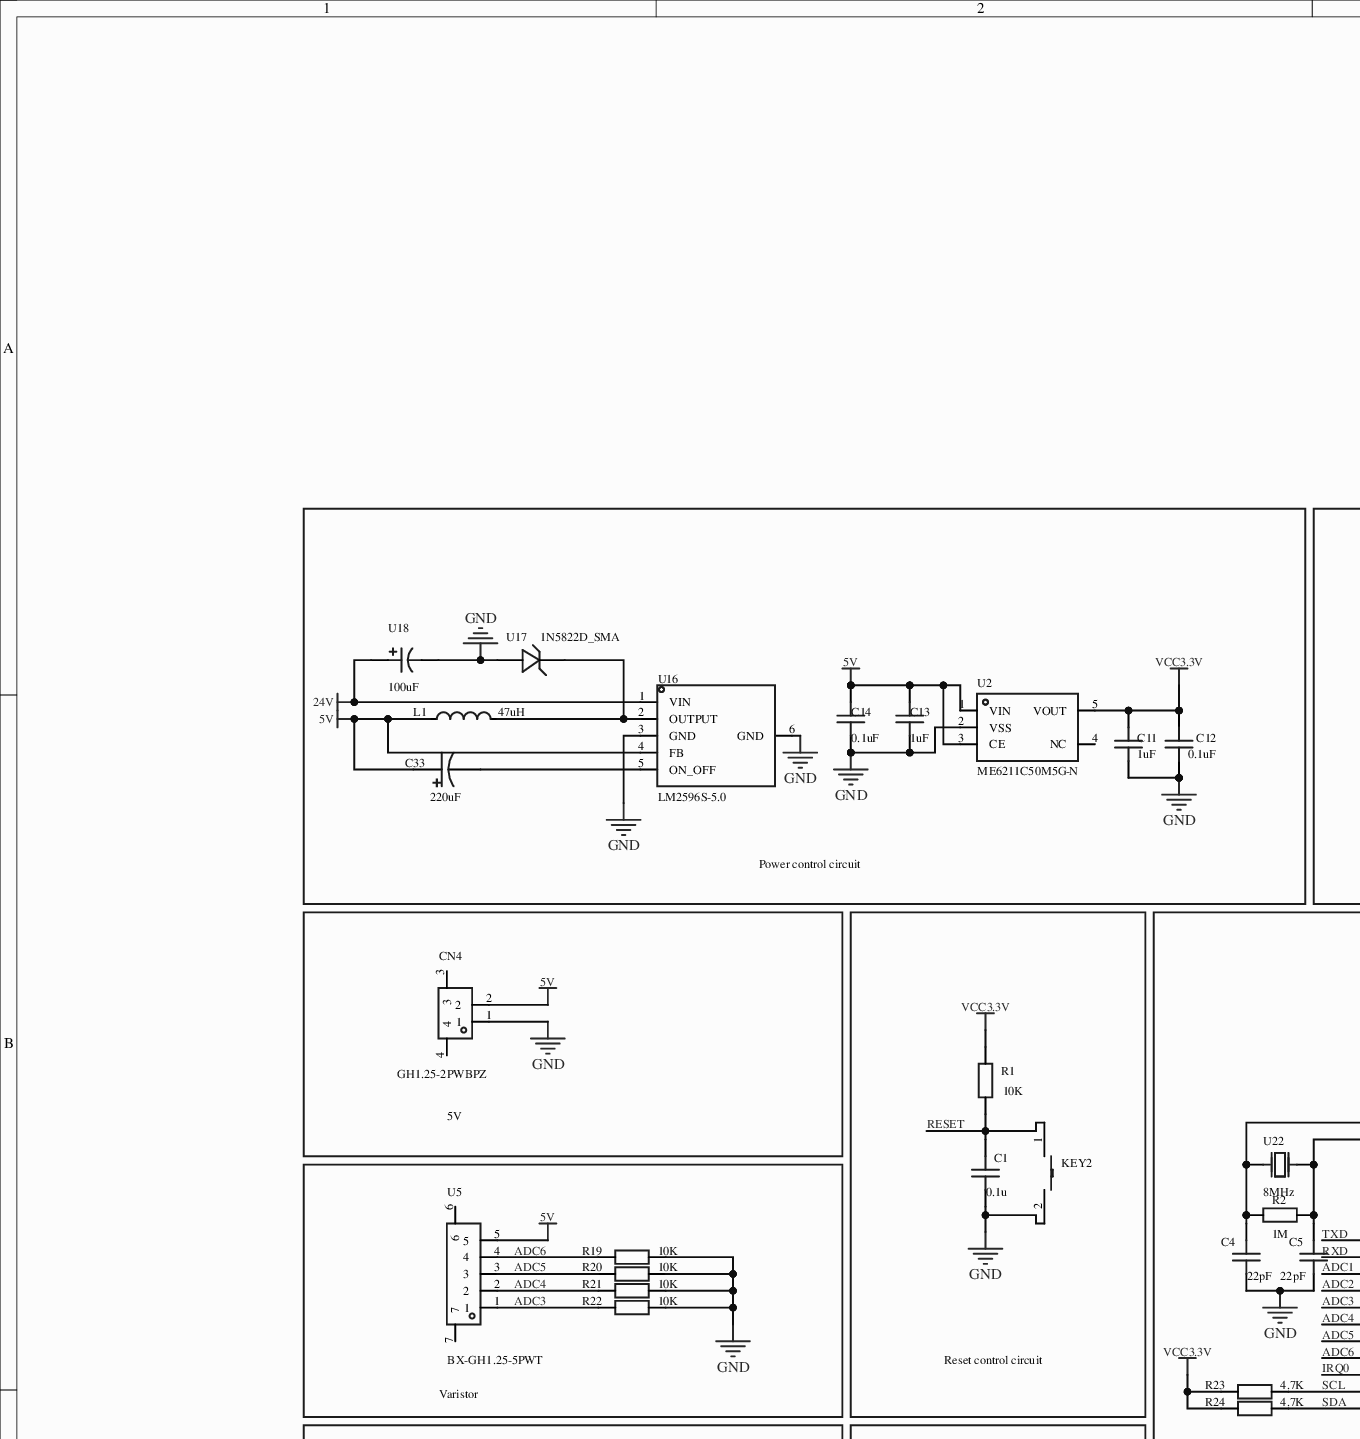
[diagram p0: MISC61403-3.schdoc, top left]
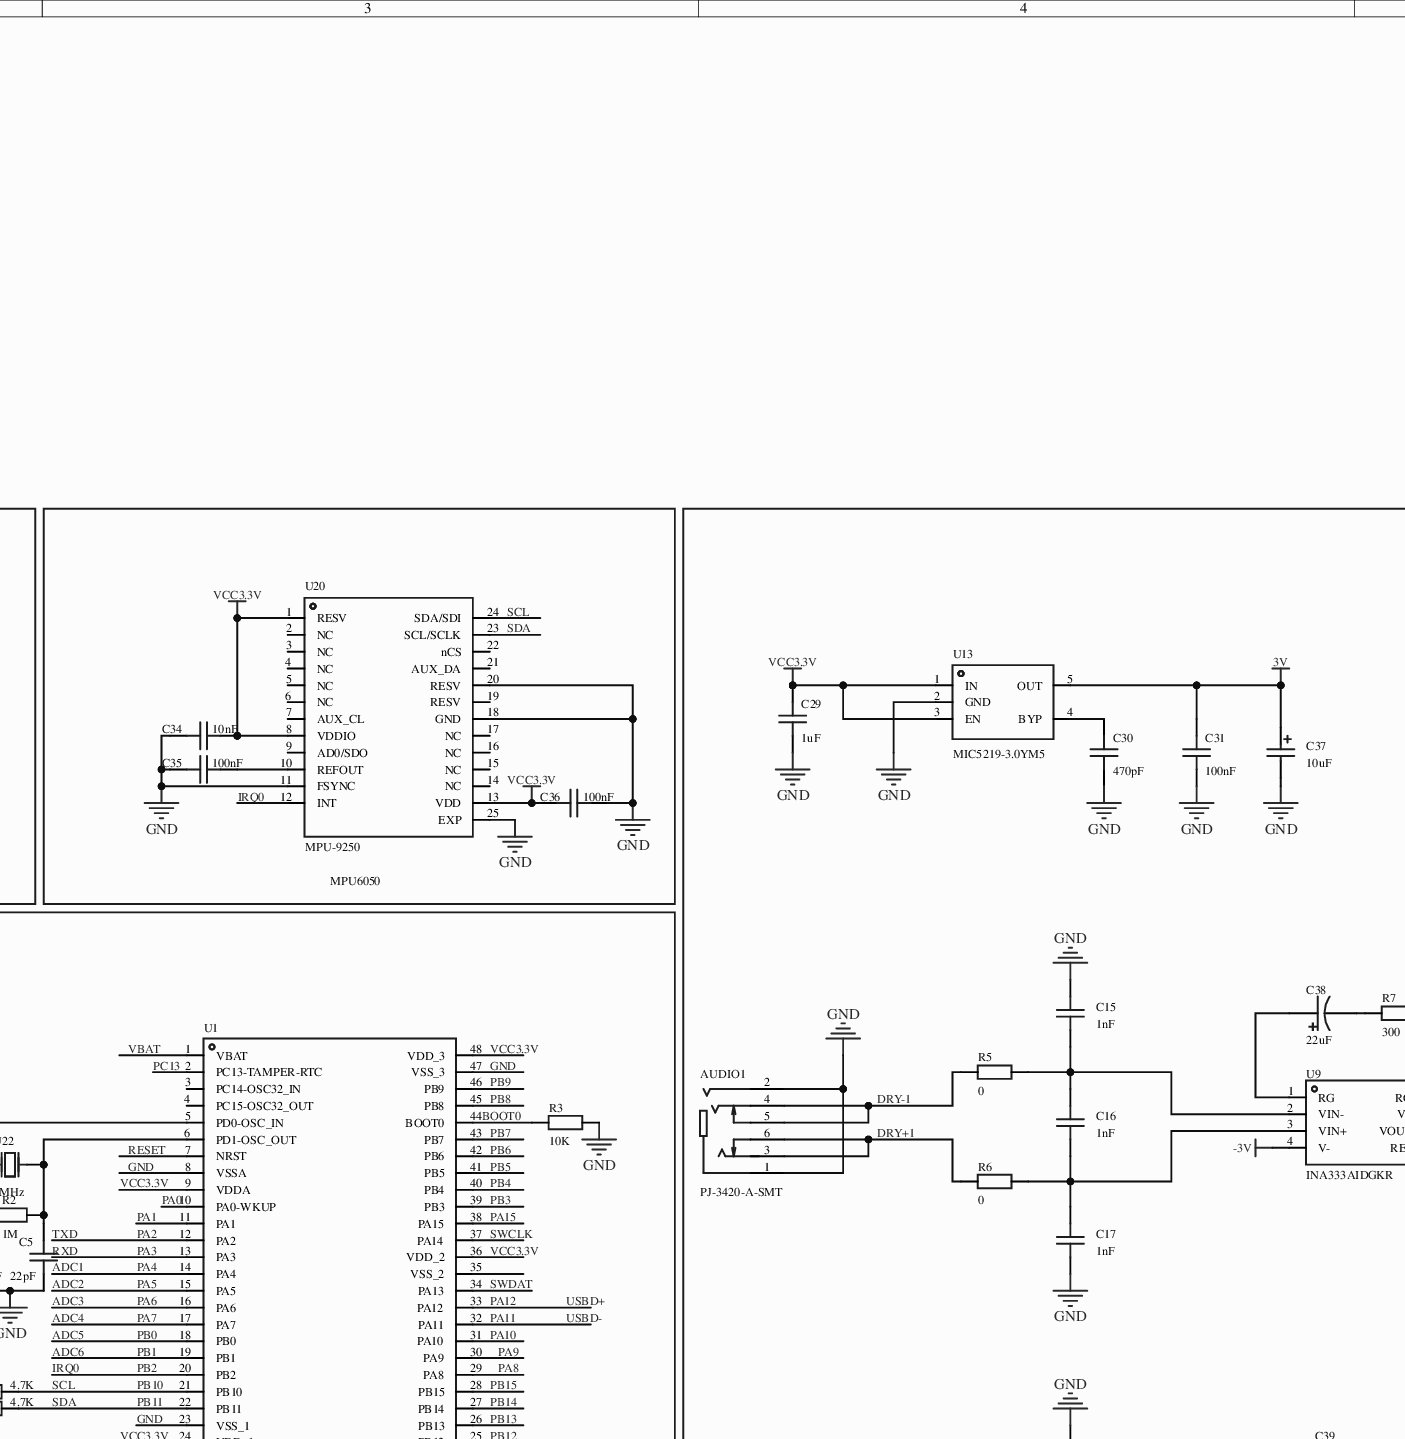
[diagram p1: MISC61403-3.schdoc, top middle]
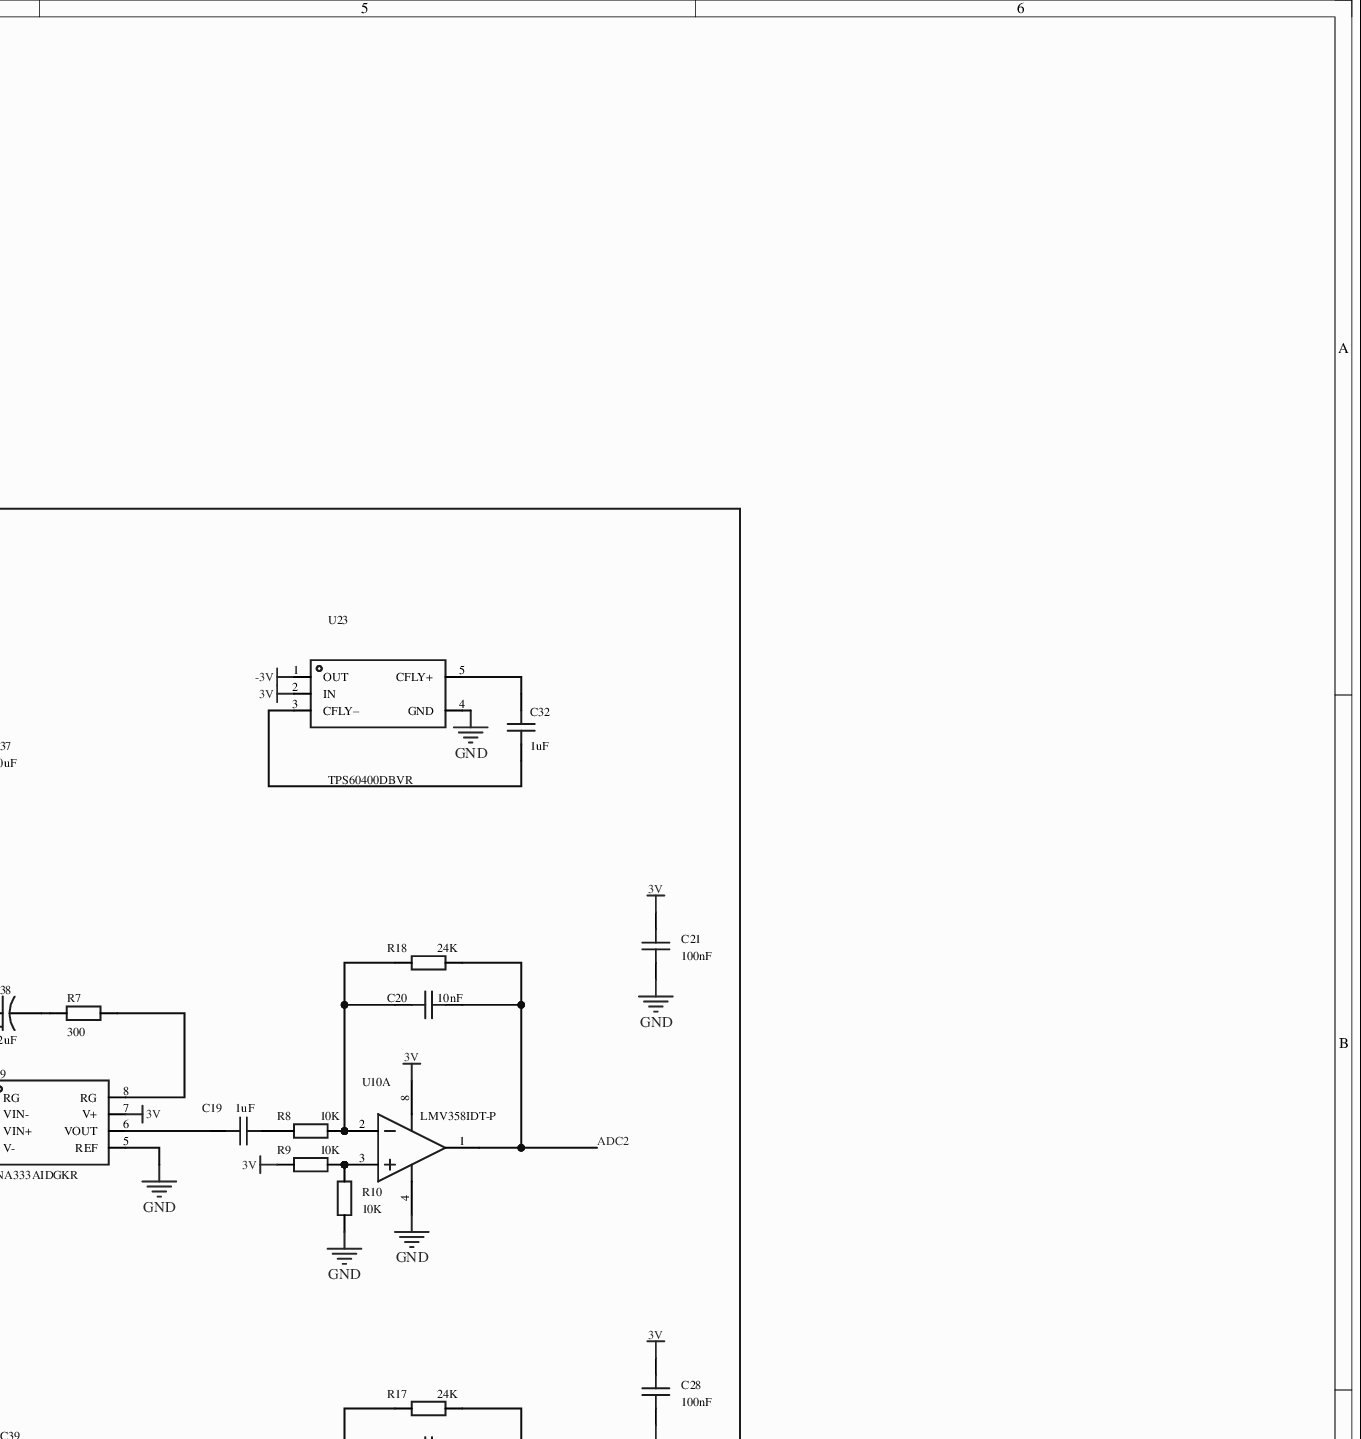
[diagram p2: MISC61403-3.schdoc, top right]
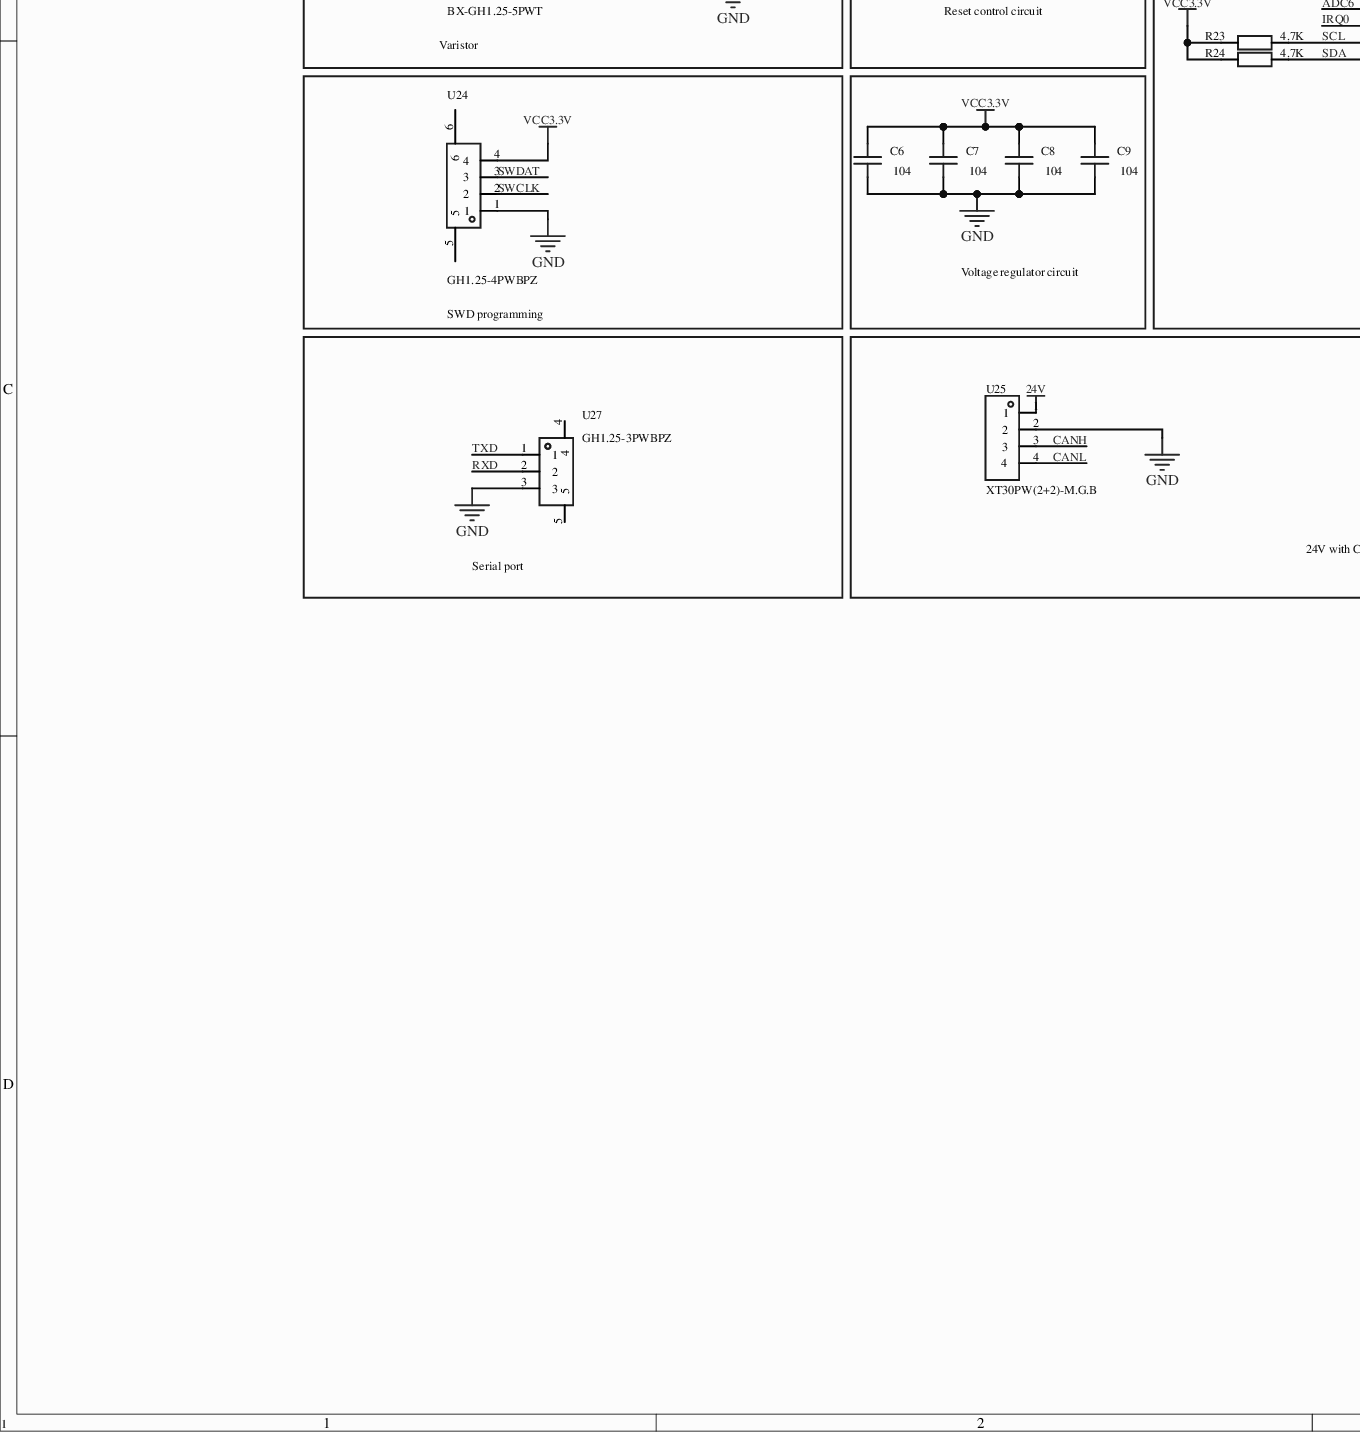
[diagram p3: MISC61403-3.schdoc, bottom left]
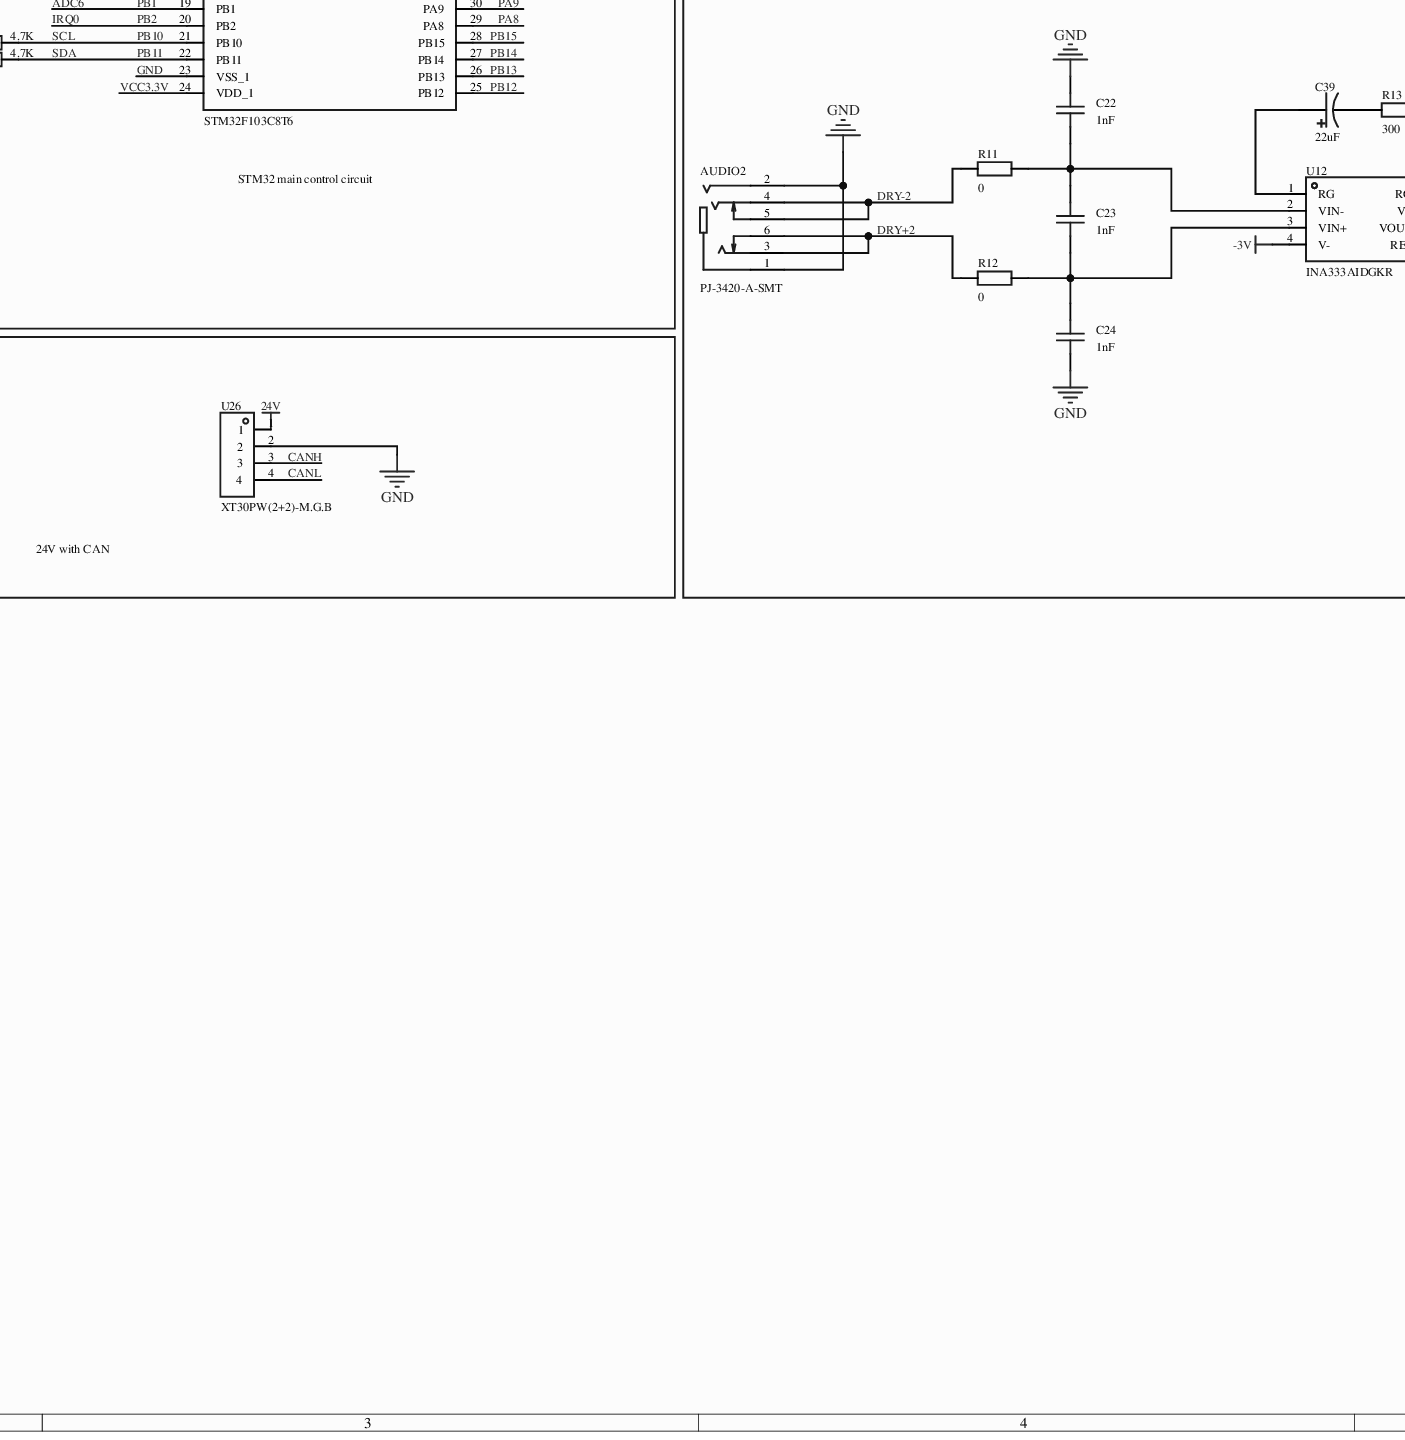
[diagram p4: MISC61403-3.schdoc, bottom middle]
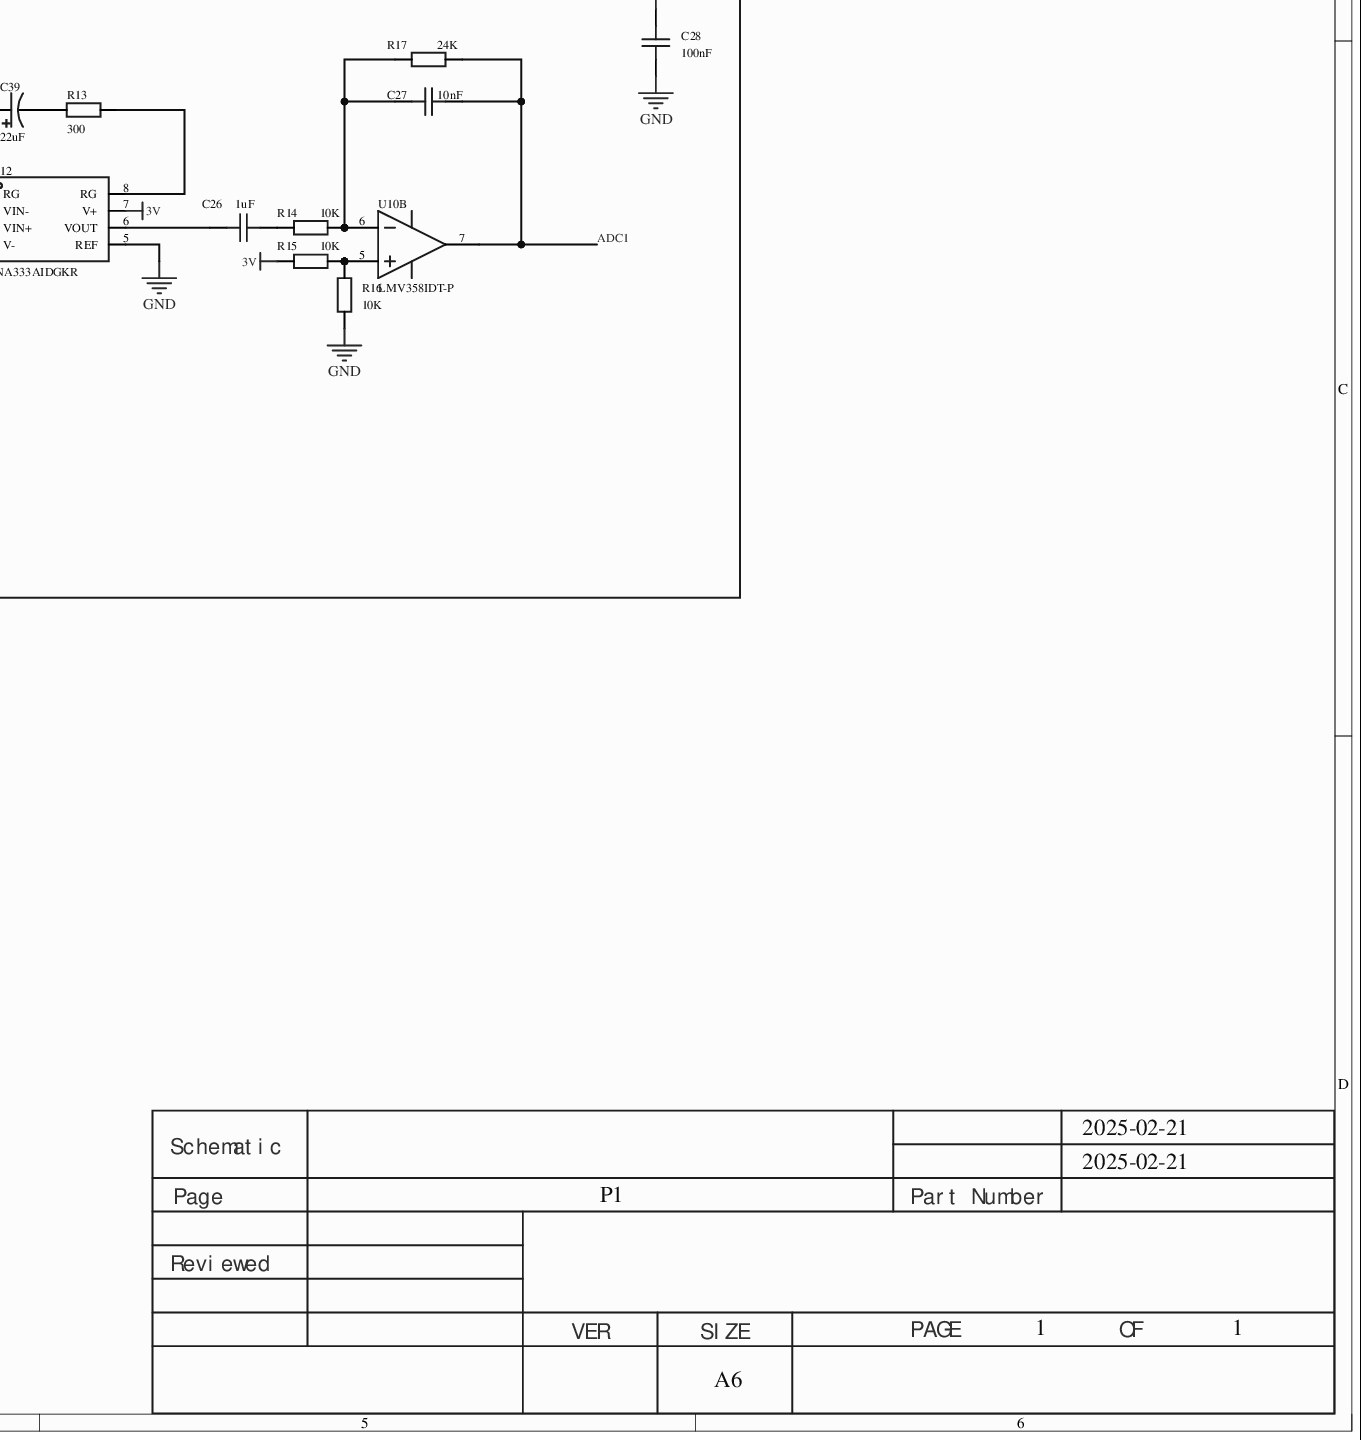
[diagram p5: MISC61403-3.schdoc, bottom right]
# Altium project MISC61403-2.PrjPcb
1 sheet, 79 parts. Net scope: global (net labels, ports and power ports of the same name join across sheets).
Board file: MISC61403.pcbdoc

## Sheet MISC61403-3.schdoc
size 594 x 419 mm; Version: V1.0; @Project Name: MISC61403; @Page Count: 1; @Update Date: 2025-02-21; @Create Date: 2025-02-21; @Schematic Name: MISC61403; @Page No: 1; @Board Name: MISC61403; @Create Time: 15:22:54; @Update Time: 18:19:48

### Parts
AUDIO1  PJ-3420-A-SMT  [AUDIO-SMD_PJ-3420-A-SMT_C319102]
AUDIO2  PJ-3420-A-SMT  [AUDIO-SMD_PJ-3420-A-SMT_C319102]
C1  0.1u  [C0603]
C4  22pF  [C0603]
C5  22pF  [C0603]
C6  104  [C0603]
C7  104  [C0603]
C8  104  [C0603]
C9  104  [C0603]
C11  1uF  [C0603]
C12  0.1uF  [C0603]
C13  1uF  [C0603]
C14  0.1uF  [C0603]
C15  1nF  [C0603]
C16  1nF  [C0603]
C17  1nF  [C0603]
C19  1uF  [C0603]
C20  10nF  [C0603]
C21  100nF  [C0603]
C22  1nF  [C0603]
C23  1nF  [C0603]
C24  1nF  [C0603]
C26  1uF  [C0603]
C27  10nF  [C0603]
C28  100nF  [C0603]
C29  1uF  [C0603]
C30  470pF  [C0603]
C31  100nF  [C0603]
C32  1uF  [C0603]
C33  220uF  [CAP-TH_BD10.0-P5.00-D1.0-FD]
C34  10nF  [C0603]
C35  100nF  [C0603]
C36  100nF  [C0603]
C37  10uF  [CAP-SMD_L3.2-W1.6-RD]
C38  22uF  [CAP-SMD_BD5.0-L5.3-W5.3-RD]
C39  22uF  [CAP-SMD_BD5.0-L5.3-W5.3-RD]
CN4  GH1.25-2PWBPZ  [CONN-SMD_GH1.25-2PWBPZ]
KEY2  TS-1101-C-W  [SW-SMD_L6.0-W3.3-LS8.0]  (value not drawn)
L1  47uH  [IND-SMD_L12.3-W12.3]
R1  10K  [R0603]
R2  1M  [R0603]
R3  10K  [R0603]
R5  0  [R0603]
R6  0  [R0603]
R7  300  [R0603]
R8  10K  [R0603]
R9  10K  [R0603]
R10  10K  [R0603]
R11  0  [R0603]
R12  0  [R0603]
R13  300  [R0603]
R14  10K  [R0603]
R15  10K  [R0603]
R16  10K  [R0603]
R17  24K  [R0603]
R18  24K  [R0603]
R19  10K  [R0603]
R20  10K  [R0603]
R21  10K  [R0603]
R22  10K  [R0603]
R23  4.7K  [R0603]
R24  4.7K  [R0603]
U1  STM32F103C8T6  [LQFP-48_L7.0-W7.0-P0.50-LS9.0-BL]
U2  ME6211C50M5G-N  [SOT-23-5_L3.0-W1.7-P0.95-LS2.8-BL]
U5  BX-GH1.25-5PWT  [CONN-SMD_5P-P1.25_BX-GH1.25-5PWT]
U9  INA333AIDGKR  [MSOP-8_L3.0-W3.0-P0.65-LS5.0-BL]
U10  LMV358IDT-P  [SOP-8_L4.9-W3.9-P1.27-LS6.0-BL]  (parts A,B of 2)
U12  INA333AIDGKR  [MSOP-8_L3.0-W3.0-P0.65-LS5.0-BL]
U13  MIC5219-3.0YM5  [SOT-23-5_L2.9-W1.6-P0.95-LS2.8-BL]
U16  LM2596S-5.0  [TO-263-5_L10.1-W8.7-P1.70-LS14.4-BR]
U17  1N5822D_SMA  [SMA_L4.3-W2.6-LS5.2-RD]
U18  100uF  [CAP-SMD_L3.5-W2.8-FD]
U20  MPU-9250  [QFN-24_L3.0-W3.0-P0.40-BL-EP]
U22  8MHz  [OSC-SMD-2P_-L5.0-W3.2]
U23  TPS60400DBVR  [SOT-23-5_L3.0-W1.7-P0.95-LS2.8-BR]
U24  GH1.25-4PWBPZ  [CONN-SMD_GH1.25-4PWBPZ]
U25  XT30PW(2+2)-M.G.B  [CONN-TH_4P-XT30PW-M]
U26  XT30PW(2+2)-M.G.B  [CONN-TH_4P-XT30PW-M]
U27  GH1.25-3PWBPZ  [CONN-SMD_GH1.25-3PWBPZ]

### Blocks framed on the sheet
Power control circuit: C11-C14 C33 L1 U2 U16-U18
MPU6050: C34-C36 U20
5V: CN4
Reset control circuit: C1 KEY2 R1
STM32 main control circuit: C4 C5 R2 R3 R23 R24 U1 U22
Varistor: R19-R22 U5
SWD programming: U24
Voltage regulator circuit: C6-C9
Serial port: U27
24V with CAN: U25 U26

### Nets
3V: C21.1 C28.1 C31.1 C37.1 R9.1 R15.1 U9.7(V+) U10.8(VDD) U12.7(V+) U13.5(OUT) U23.2(IN)
5V: C13.2 C14.2 C33.1 CN4.2 L1.1 U2.1(VIN) U2.3(CE) U5.5 U16.4(FB)
24V: U16.1(VIN) U18.1 U25.1 U26.1
-3V: U9.4(V-) U12.4(V-) U23.1(OUT)
GND: AUDIO1.1 AUDIO1.2 AUDIO2.1 AUDIO2.2 C1.1 C4.1 C5.1 C6.1 C7.1 C8.1 C9.1 C11.1 C12.1 C13.1 C14.1 C15.2 C17.1 C21.2 C22.2 C24.1 C28.2 C29.2 C30.2 C31.2 C34.2 C35.2 C36.2 C37.2 CN4.1 KEY2.2 R3.2 R10.1 R16.1 R19.1 R20.1 R21.1 R22.1 U1.8(VSSA) U1.23(VSS_1) U1.47(VSS_3) U2.2(VSS) U9.5(REF) U10.4(VSS) U12.5(REF) U13.2(GND) U16.3(GND) U16.6(GND) U17.2(A) U18.2 U20.11(FSYNC) U20.18(GND) U20.20(RESV) U20.25(EXP) U23.4(GND) U24.1 U25.2 U26.2 U27.3
VCC3.3V: C6.2 C7.2 C8.2 C9.2 C11.2 C12.2 C29.1 C34.1 C36.1 R1.2 R23.1 R24.1 U1.9(VDDA) U1.24(VDD_1) U1.36(VDD_2) U1.48(VDD_3) U2.5(VOUT) U13.1(IN) U13.3(EN) U20.1(RESV) U20.8(VDDIO) U20.13(VDD) U24.4
ADC1: C27.1 R17.2 U1.14(PA4) U10.7(OUTB)  [also labelled PA4]
ADC2: C20.1 R18.2 U1.15(PA5) U10.1(OUTA)  [also labelled PA5]
ADC3: R22.2 U1.16(PA6) U5.1  [also labelled PA6]
ADC4: R21.2 U1.17(PA7) U5.2  [also labelled PA7]
ADC5: R20.2 U1.18(PB0) U5.3  [also labelled PB0]
ADC6: R19.2 U1.19(PB1) U5.4  [also labelled PB1]
BOOT0: R3.1 U1.44(BOOT0)
CANH: U25.3 U26.3
CANL: U25.4 U26.4
DRY+1: AUDIO1.3 AUDIO1.6 R6.1
DRY+2: AUDIO2.3 AUDIO2.6 R12.1
DRY-1: AUDIO1.4 AUDIO1.5 R5.1
DRY-2: AUDIO2.4 AUDIO2.5 R11.1
IRQ0: U1.20(PB2) U20.12(INT)  [also labelled PB2]
PA0: U1.10(PA0-WKUP)
PA1: U1.11(PA1)
PA2: U1.12(PA2) U27.1  [also labelled TXD]
PA3: U1.13(PA3) U27.2  [also labelled RXD]
PA8: U1.29(PA8)
PA9: U1.30(PA9)
PA10: U1.31(PA10)
PA11: U1.32(PA11)  [also labelled USBD-]
PA12: U1.33(PA12)  [also labelled USBD+]
PA15: U1.38(PA15)
PB3: U1.39(PB3)
PB4: U1.40(PB4)
PB5: U1.41(PB5)
PB6: U1.42(PB6)
PB7: U1.43(PB7)
PB8: U1.45(PB8)
PB9: U1.46(PB9)
PB10: R23.2 U1.21(PB10) U20.24(SDA/SDI)  [also labelled SCL]
PB11: R24.2 U1.22(PB11) U20.23(SCL/SCLK)  [also labelled SDA]
PB12: U1.25(PB12)
PB13: U1.26(PB13)
PB14: U1.27(PB14)
PB15: U1.28(PB15)
PC13: U1.2(PC13-TAMPER-RTC)
RESET: C1.2 KEY2.1 R1.1 U1.7(NRST)
SWCLK: U1.37(PA14) U24.2
SWDAT: U1.34(PA13) U24.3
VBAT: U1.1(VBAT)
NetC4_2: C4.2 R2.1 U1.5(PD0-OSC_IN) U22.1(OSC1)
NetC5_2: C5.2 R2.2 U1.6(PD1-OSC_OUT) U22.2(OSC2)
NetC15_1: C15.1 C16.2 R5.2 U9.2(VIN-)
NetC16_1: C16.1 C17.2 R6.2 U9.3(VIN+)
NetC19_1: C19.1 R8.1
NetC19_2: C19.2 U9.6(VOUT)
NetC20_2: C20.2 R8.2 R18.1 U10.2(INA-)
NetC22_1: C22.1 C23.2 R11.2 U12.2(VIN-)
NetC23_1: C23.1 C24.2 R12.2 U12.3(VIN+)
NetC26_1: C26.1 R14.1
NetC26_2: C26.2 U12.6(VOUT)
NetC27_2: C27.2 R14.2 R17.1 U10.6(INB-)
NetC30_1: C30.1 U13.4(BYP)
NetC32_1: C32.1 U23.5(CFLY+)
NetC32_2: C32.2 U23.3(CFLY–)
NetC33_2: C33.2 U16.5(ON_OFF)
NetC35_1: C35.1 U20.10(REFOUT)
NetC38_1: C38.1 U9.1(RG)
NetC38_2: C38.2 R7.1
NetC39_1: C39.1 U12.1(RG)
NetC39_2: C39.2 R13.1
NetL1_2: L1.2 U16.2(OUTPUT) U17.1(C)
NetR7_2: R7.2 U9.8(RG)
NetR9_2: R9.2 R10.2 U10.3(INA+)
NetR13_2: R13.2 U12.8(RG)
NetR15_2: R15.2 R16.2 U10.5(INB+)

Not connected (* = marked no-connect by the designer): CN4 3 4; U1 3(PC14-OSC32_IN)* 4(PC15-OSC32_OUT)* 35(VSS_2); U2 4(NC)*; U5 6 7; U20 2(NC)* 3(NC)* 4(NC)* 5(NC)* 6(NC)* 7(AUX_CL)* 9(AD0/SDO)* 14(NC)* 15(NC)* 16(NC)* 17(NC)* 19(RESV)* 21(AUX_DA)* 22(nCS)*; U24 5 6; U27 4 5

### Notes on the sheet
- 2025-02-21
- Schematic
- Page
- P1
- Part Number
- Reviewed
- VER
- SIZE
- A6
- PAGE
- 1
- OF

### Library data of the parts
AUDIO1 AUDIO2 = PJ-3420-A-SMT: Connector type:3.5mm headphone jack;Rated current:500mA;Rated voltage:30V;Operating temperature range:-20℃~+70℃;Soldering temperature (max):235℃;; Manufacturer: XKB Connectivity(中国星坤); Symbol: PJ-3537-X; AddInBom: yes; ModelId: f64a06432b8d4649a6d00824f883fe68; ModelTransform: 551.18,326.771,0,0,0,0,-70.157,-0.004,-23.622; Current Rating (Max): 500mA; Voltage Rating (Max): 30V; Soldering Temperature(Max): 235℃; Device: PJ-3420-A-SMT; LCSC Part Name: 3.5mm耳机座; SupplierPart: C319102; ManufacturerPart: PJ-3420-A-SMT; Supplier Footprint: SMD; JLCPCB Part Class: Extended library; Datasheet: https://atta.szlcsc.com/upload/public/pdf/source/20211015/FA11597DF53DC331FB6A72D64BA50234.pdf; Supplier: LCSC; ConvertToPcb: yes; FootprintName: AUDIO-SMD_PJ-3420-A-SMT_C319102; ModelName: AUDIO-SMD_PJ-3420-A-SMT_C319102; Connector Type: 3.5mm headphone jack; Operating Temperature Range: -20℃~+70℃
C1 C4-C9 C11-C17 C19-C24 C26-C32 C34-C36 = CAP_0603: ConvertToPcb: yes; SymbolName: CapAcitance; ModelId: ac125912035d415993ca9572d50418b1; ModelName: C0603_L1.6-W0.8-H0.8; ModelTransform: 62.992,31.496,0,0,0,0,0,0,0; Device: CAP_0603; AddInBom: yes; Supplier Footprint: 0603; FootprintName: C0603
  C1: Value: 0.1u
  C4 C5: Value: 22pF
  C6-C9: Value: 104
  C11 C13 C19 C26 C29 C32: Value: 1uF
  C12 C14: Value: 0.1uF
  C15-C17 C22-C24: Value: 1nF
  C20 C27 C34: Value: 10nF
  C21 C28 C31 C35 C36: Value: 100nF
  C30: Value: 470pF
C33 = EEUFC1V221B: Capacitance:220uF;Tolerance:±20%;Rated voltage:35V;Ripple current:755mA@100kHz;Equivalent series resistance:90mΩ@100kHz;; Manufacturer: PANASONIC(松下); AddInBom: yes; ModelId: 6ce78ce5315348e095d700085da75e48; ModelName: CAP-TH_D10.0-H16.0-P5.00; ModelTransform: 394.094,393.72252,0,0,0,0,0,0,-137.795; Tolerance: ±20%; Rated Voltage: 35V; φD: 10mm; L: 12.5mm; Lifetime @ Temp: 3000hrs@105℃; Symbol: EEUFC1V221B; Device: EEUFC1V221B; LCSC Part Name: 220uF ±20% 35V; SupplierPart: C178681; ManufacturerPart: EEUFC1V221B; Supplier Footprint: 插件,D10xL12.5mm; JLCPCB Part Class: Extended library; Datasheet: https://atta.szlcsc.com/upload/public/pdf/source/20181222/C178681_6E15EF82E6D495A72D0777BE3B4ACA7A.pdf; Supplier: LCSC; ConvertToPcb: yes; FootprintName: CAP-TH_BD10.0-P5.00-D1.0-FD; Value: 220uF; Ripple Current: 755mA@100kHz; Equivalent Series Resistance(ESR): 90mΩ@100kHz; Lead Spacing: 5mm; Operating Temperature: -55℃~+105℃
C37 = CA45-A-16V-10uF-K: Capacitance:10uF;Tolerance:±10%;Rated voltage:16V;Equivalent series resistance:10Ω@100kHz;; Manufacturer: CEC(振华新云); AddInBom: yes; ModelId: d42b6f9952ad429a883ac5dd55ff7452; ModelName: CASE-A_L3.2-W1.6-H1.6; ModelTransform: 125.984,62.992,0,0,0,0,0,0,0; Tolerance: ±10%; Rated Voltage: 16V; Symbol: CA45-A-16V-10UF-K; Device: CA45-A-16V-10uF-K; LCSC Part Name: 10uF ±10% 16V; SupplierPart: C128254; ManufacturerPart: CA45-A-16V-10uF-K; Supplier Footprint: CASE-A-3216; JLCPCB Part Class: Extended library; Datasheet: https://atta.szlcsc.com/upload/public/pdf/source/20170914/C128254_1505359752472967905.pdf; Supplier: LCSC; ConvertToPcb: yes; FootprintName: CAP-SMD_L3.2-W1.6-RD; Value: 10uF; Equivalent Series Resistance(ESR): 10Ω@100kHz; Operating Temperature: -55℃~+125℃
C38 C39 = VKMB1001H220MV: Capacitance:22uF;Tolerance:±20%;Rated voltage:50V;Ripple current:238mA@100kHz;Equivalent series resistance:-;; Manufacturer: Ymin(永铭); AddInBom: yes; ModelId: 055d55eb99d5406da0ea9a7b573ef45c; ModelName: CAP-SMD_L5.3-W5.3-H5.3-LS5.9; ModelTransform: 208.661,232.283,0,270,0,0,0,0,0; Tolerance: ±20%; Rated Voltage: 50V; φD: 5mm; L: 10mm; Lifetime @ Temp: 7000hrs@105℃; Symbol: VKMB1001H220MV; Device: VKMB1001H220MV; LCSC Part Name: 22uF ±20% 50V; SupplierPart: C487355; ManufacturerPart: VKMB1001H220MV; Supplier Footprint: SMD,D5xL10mm; JLCPCB Part Class: Extended library; Datasheet: https://atta.szlcsc.com/upload/public/pdf/source/20200220/C487598_2A147BEF594D77F42D2799F3121C99E1.pdf; Supplier: LCSC; ConvertToPcb: yes; FootprintName: CAP-SMD_BD5.0-L5.3-W5.3-RD; Value: 22uF; Ripple Current: 238mA@100kHz; Equivalent Series Resistance(ESR): -; Operating Temperature: -55℃~+105℃
CN4 = GH1.25-2PWBPZ: Manufacturer: BOOMELE(博穆精密); AddInBom: yes; ModelId: 3468b1afc40c4447814fbf6372d6c8fd; ModelTransform: 226.7712,196.85,0,0,0,0,0,-12.047,0; Symbol: GH1.25-2PWBPZ; Device: GH1.25-2PWBPZ; LCSC Part Name: GH1.25-2P卧贴编带; SupplierPart: C2829251; ManufacturerPart: GH1.25-2PWBPZ; Supplier Footprint: -; JLCPCB Part Class: Extended library; Datasheet: https://atta.szlcsc.com/upload/public/pdf/source/20211125/08A09A4909F58AF780B71FE423A00F7E.pdf; Supplier: LCSC; ConvertToPcb: yes; FootprintName: CONN-SMD_GH1.25-2PWBPZ; ModelName: CONN-SMD_GH1.25-2PWBPZ
KEY2 = TS-1101-C-W: Contact current:50mA;Rated voltage (DC):12V;Insulation resistance:-;Circuit structure:SPST;Mounting style:Vertical SMT;Button shape:Rectangular button;Button/cap color:White;With lamp:None;Actuation force:260gf;Mechanical life:50000;Operating temperature:-30℃~+85℃;Switch length:6mm;Switch width:3.6mm;Switch height:2.5mm;With bracket:No;; Manufacturer: XKB Connectivity(中国星坤); AddInBom: yes; ModelId: b2f4ea9f0afc4b0786d53dba66ceb9e4; ModelName: SW-SMD_L6.0-W3.3-H5-LS8.0; ModelTransform: 314.96,129.921,0,0,0,0,0,0,0; Contact Current: 50mA; Voltage Rating (DC): 12V; Circuit: SPST; Actuator/Cap Color: White; With Lamp: None; Operating Force: 260gf; Mechanical Life: 50000; Switch Length: 6mm; Switch Width: 3.6mm; Switch Height: 2.5mm; Strike Gundam: No; Device: TS-1101-C-W; Symbol: TS-1101-C-W; LCSC Part Name: TS-1101-C-W 一型3*6*2.5有白ZD b拉伸白色按键 卷装; SupplierPart: C318938; ManufacturerPart: TS-1101-C-W; Supplier Footprint: SMD; JLCPCB Part Class: Extended Part; Datasheet: https://atta.szlcsc.com/upload/public/pdf/source/20200227/C318938_C2E53B1EEDE37D980A33616AC086DE53.pdf; Supplier: LCSC; ConvertToPcb: yes; FootprintName: SW-SMD_L6.0-W3.3-LS8.0; Insulation Resistance: -; Mounting Style: Vertical SMT; Actuator Style: Rectangular button; Operating Temperature: -30℃~+85℃
L1 = CDRH127N-470M: Inductance:47uH;Tolerance:±20%;Rated current:-;Saturation current (Isat):-;; Manufacturer: MINGSTAR(登壹); AddInBom: yes; ModelId: 1430fda232714ed3b12b8476f42d35be; ModelName: SMD-PIND_L12.5-W12.5-H8.0; ModelTransform: 494.75925,492.125,0,0,0,0,-0.005,0,0; Tolerance: ±20%; Symbol: CDRH127N-470M; Device: CDRH127N-470M; LCSC Part Name: 47uH ±20%; SupplierPart: C962356; ManufacturerPart: CDRH127N-470M; Supplier Footprint: SMD,12.3x12.3mm; JLCPCB Part Class: Extended library; Datasheet: https://atta.szlcsc.com/upload/public/pdf/source/20201218/C962356_DBB80431F2386180CBD0A67FB703DD56.pdf; Supplier: LCSC; ConvertToPcb: yes; FootprintName: IND-SMD_L12.3-W12.3; Value: 47uH; Rated Current: -; Saturation Current (Isat): -; DC Resistance (DCR): -; Ratings: -
R1 R2 R19-R22 = Res_0603: Symbol: Resistor; ConvertToPcb: yes; ModelId: 6bd5cd867e9542ebae21caaf5d2d4c4d; ModelTransform: 31.8897,63.7794,0,90,0,0,0,0,0; Device: Res_0603; AddInBom: yes; Supplier Footprint: 0603; FootprintName: R0603; ModelName: R0603
  R1 R19-R22: Value: 10K
  R2: Value: 1M
R3 R5-R18 R23 R24 = Res_0603: ConvertToPcb: yes; SymbolName: Resistor; ModelId: fc143cca1e79419f9cd78b61e9279f08; ModelTransform: 31.8897,63.7794,0,90,0,0,0,0,0; Device: Res_0603; AddInBom: yes; Supplier Footprint: 0603; FootprintName: R0603; ModelName: R0603
  R3 R8-R10 R14-R16: Value: 10K
  R5 R6 R11 R12: Value: 0
  R7 R13: Value: 300
  R17 R18: Value: 24K
  R23 R24: Value: 4.7K
U1 = STM32F103C8T6: CPU core:ARM Cortex-M3;CPU max frequency:72MHz;Program storage capacity:64KB;Program memory type:FLASH;Total RAM:20KB;GPIO port count:37;ADC (bits):12bit;Operating temperature range:-40℃~+85℃;; Manufacturer: ST(意法半导体); AddInBom: yes; ModelId: 093be70396ff421eb2cdb946d5311efc; ModelName: LQFP-48_L7.0-W7.0-H1.4-LS9.0-P0.50; ModelTransform: 354.331,354.331,0,0,0,0,0,0,0; CPU Maximum Speed: 72MHz; Operating Voltage Range: 2V~3.6V; Program Storage Size: 64KB; Program Memory Type: FLASH; RAM Size: 20KB; GPIO Ports Number: 37; ADC (Bit): 12bit; Peripheral/Function: Watchdog; DMA; Watchdog; On-chip temperature sensor; Device: STM32F103C8T6; Symbol: STM32F103C8T6; LCSC Part Name: ARM Cortex-M3 72MHz MSL=3; SupplierPart: C8734; ManufacturerPart: STM32F103C8T6; Supplier Footprint: LQFP-48(7x7); JLCPCB Part Class: Basic Part; Datasheet: https://atta.szlcsc.com/upload/public/pdf/source/20220812/8363ACEC51AD55ECEB84799464F7CB85.pdf; Supplier: LCSC; ConvertToPcb: yes; FootprintName: LQFP-48_L7.0-W7.0-P0.50-LS9.0-BL; CPU Core: ARM Cortex-M3; EEPROM: 64KB; DAC (Bit): -; PWM (Bit): -; Universal Serial Bus: -; Internal Comparator: -; communication protocol: -; Watchdog: -; Real-Time Clock: -; Infrared Data Association: -; Low-Voltage Detect: -; CCP Capture/Compare: -; Secure Digital Input and Output: -; Direct Memory Access: -; Internal Oscillator: Yes; Operating Temperature Range: -40℃~+85℃
U2 = ME6211C50M5G-N: -; Manufacturer: MICRONE(南京微盟); AddInBom: yes; ModelId: 0a2a1b8f50944f73965918ad6e5fe167; ModelName: SOT-23-5_L2.9-W1.6-H1.1-LS2.8-P0.95; ModelTransform: 118.60433,114.173,0,90,0,0,0.0005,0.0005,0; Device: ME6211C50M5G-N; Symbol: ME6211C50M5G-N; LCSC Part Name: ME6211C50M5G-N; SupplierPart: C236670; ManufacturerPart: ME6211C50M5G-N; Supplier Footprint: SOT-23-5; JLCPCB Part Class: Extended Part; Datasheet: https://atta.szlcsc.com/upload/public/pdf/source/20180709/C236670_CE73D272779D26EBD8CFC2246415DB9C.pdf; Supplier: LCSC; ConvertToPcb: yes; FootprintName: SOT-23-5_L3.0-W1.7-P0.95-LS2.8-BL
U5 = BX-GH1.25-5PWT: Pin structure:1x5P;Pitch:1.25mm;Mounting style:Horizontal SMT;Reference series:GH;Total pins:5P;Rows:1;Pins per row:5;Row spacing:-;Rated current:1A;Contact material:Phosphor bronze;Contact plating:Tin;Operating temperature:-25℃~+85℃;; Manufacturer: Bossie(博锡); AddInBom: yes; ModelId: ba7089444aff4848bfc66fe8b1f6662a; ModelTransform: 374.015,190.9445,0,0,0,0,0,-17.008,0; Pins Structure: 1x5P; Pitch: 1.25mm; Reference Series: GH; Number of PINs Per Row: 5; Current Rating: 1A; Voltage Rating: 125V; Plastic Material: LCP; Supplementary Features: Auxiliary solder tabs; Z-Height of the Board: 4.35mm; X-Length of Bottom Edge on Board (Spacing Line): 9.5mm; Y-Width of Bottom Edge on Board: 5mm; Symbol: BX-GH1.25-5PWT; Device: BX-GH1.25-5PWT; LCSC Part Name: 1x5P 间距:1.25mm 卧贴 系列:GH; SupplierPart: C18077721; ManufacturerPart: BX-GH1.25-5PWT; Supplier Footprint: SMD,P=1.25mm,卧贴; JLCPCB Part Class: Extended library; Datasheet: https://atta.szlcsc.com/upload/public/pdf/source/20231017/9CBEA5754A21F666D6038AF11B67503D.pdf; Supplier: LCSC; ConvertToPcb: yes; FootprintName: CONN-SMD_5P-P1.25_BX-GH1.25-5PWT; ModelName: CONN-SMD_5P-P1.25_BX-GH1.25-5PWT; Mounting Type: Horizontal SMT; Number of Pins: 5P; Number of Rows: 1; Row Spacing: -; Contact Material: Phosphor bronze; Contact Plating: Tin; Operating Temperature: -25℃~+85℃; Flame Retardant Rating: -; Color: Beige
U9 U12 = INA333AIDGKR: Amplifier count:Single;Input bias current (Ib):70pA;Input offset voltage (Vos):10uV;Slew rate (SR):0.16V/us;Bandwidth (-3dB):150kHz;Rail-to-rail:-;; Manufacturer: TI(德州仪器); AddInBom: yes; ModelId: 1de5a054e9244f539c6db8238d445f94; ModelTransform: 118.11,196.85,0,0,0,0,0,0,0; Number of Circuits: Single; Current - Input Bias(Ib): 70pA; Voltage - Input Offset(Vos): 10uV; -3db Bandwidth: 150kHz; Symbol: INA333AIDGKR; Device: INA333AIDGKR; LCSC Part Name: INA333AIDGKR; SupplierPart: C19450; ManufacturerPart: INA333AIDGKR; Supplier Footprint: MSOP-8; JLCPCB Part Class: Extended library; Supplier: LCSC; ConvertToPcb: yes; FootprintName: MSOP-8_L3.0-W3.0-P0.65-LS5.0-BL; ModelName: MSOP-8_L3.0-W3.0-P0.65-LS5.0-BL; Slew Rate(SR): 0.16V/us; Rail to Rail: -; Output Type: -; Operating Temperature: -40℃~+125℃
U10 = LMV358IDT-P: Rail-to-rail:Rail-to-rail input, rail-to-rail output;Gain bandwidth product (GBP):1MHz;Input offset voltage (Vos):5mV;Slew rate (SR):0.6V/us;; Manufacturer: TECH PUBLIC(台舟); Relevance: []; AddInBom: yes; ModelId: 75c24a7891ee4dd6bdac16a7163ff87e; ModelName: SOP-8_L4.9-W3.9-P1.27-LS6.0-BL-1; ModelTransform: 192.913,236.22,0,0,0,0,0,0,0; Maximum Power Supply Range (Vdd-Vss): 5.5V; Gain Bandwidth Product(GBP): 1MHz; Voltage - Input Offset(Vos): 5mV; Input Offset Voltage Drift (Vos TC): 2uV/℃; Noise density(eN): 20nV/√Hz@10kHz; Common Mode Rejection Ratio (CMRR): 65dB; Symbol: LMV358IDT-P; Device: LMV358IDT-P; LCSC Part Name: 运算放大器; SupplierPart: C2937045; ManufacturerPart: LMV358IDT-P; Supplier Footprint: SOP-8; JLCPCB Part Class: Extended library; Datasheet: https://atta.szlcsc.com/upload/public/pdf/source/20220105/C7B48EA4CDD740C90F101FA28962CA5C.pdf; Supplier: LCSC; ConvertToPcb: yes; FootprintName: SOP-8_L4.9-W3.9-P1.27-LS6.0-BL; Rail to Rail: Rail-to-rail input, rail-to-rail output; Slew Rate(SR): 0.6V/us
U13 = MIC5219-3.0YM5-TR: Output type:Fixed;Max input voltage:12V;Output voltage:3V;Max output current:500mA;Power supply ripple rejection (PSRR):75dB@(120Hz);Output polarity:Positive;; Manufacturer: MICROCHIP(美国微芯); AddInBom: yes; ModelId: 018c57e721114987ae90467fe9f1d259; ModelTransform: 114.96,110.236,0,0,0,0,0,0,0; Output Type: Fixed; Maximum Input Voltage: 12V; Output Voltage: 3V; MAX Output Current: 500mA; Dropout Voltage: 600mV@(500mA); standby current: 8uA; Number of Outputs: 1; Symbol: MIC5219-3.0YM5-TR; Manufacturer Part: MIC5219-3.0YM5; Device: MIC5219-3.0YM5-TR; LCSC Part Name: 输入12V 输出3V 500mA; SupplierPart: C145375; Supplier Footprint: SOT-23-5; JLCPCB Part Class: Extended library; Datasheet: https://atta.szlcsc.com/upload/public/pdf/source/20171212/C145689_15130637213801177745.pdf; Supplier: LCSC; ConvertToPcb: yes; FootprintName: SOT-23-5_L2.9-W1.6-P0.95-LS2.8-BL; ModelName: SOT-23-5_L2.9-W1.6-P0.95-LS2.8-BL; Power Supply Rejection Ratio (PSRR): 75dB@(120Hz); Operating Temperature: -40℃~+125℃; Output Polarity: Positive
U16 = LM2596S-5.0: Function type:Step-down;Output type:Fixed;Operating voltage:4.5V~30V;Output voltage:5V;Output current:3A;; Manufacturer: Slkor(萨科微); Symbol: LM2596S-5.0_C2980820; AddInBom: yes; ModelId: 5538f873629a4091a60928eafa887b89; ModelName: TO-263-5_L10.13-W8.74-P1.70-LS14.38-BR; ModelTransform: 405.511,562.20364,0,90,0,0,-52.721,0.002,0; Output Type: Fixed; Output Voltage: 5V; Output Current: 3A; Switching Frequency: 150kHz; Synchronous Rectification: No; Number of Outputs: 1; Topology: Buck; Quiescent Current (Iq): 2mA; Switch tube (built-in/external): Built-in; Device: LM2596S-5.0; LCSC Part Name: 3A 150KHz 固定频率 PWM DC-DC 降压稳压器; SupplierPart: C2980820; ManufacturerPart: LM2596S-5.0; Supplier Footprint: TO-263-5; JLCPCB Part Class: Extended library; Datasheet: https://atta.szlcsc.com/upload/public/pdf/source/20240712/15D090E1E62A66287317EE8B2A6B0426.pdf; Supplier: LCSC; ConvertToPcb: yes; FootprintName: TO-263-5_L10.1-W8.7-P1.70-LS14.4-BR; Function: Step-down; Input Voltage: 4.5V~30V; Operating Temperature: -40℃~+125℃
U17 = 1N5822D_SMA: AddInBom: yes; ModelId: 7ed2c9d0a4a74bbdbba07ab4052caf5b; ModelTransform: 185.039,102.362,0,0,0,0,0,0,0; Symbol: 1N5822D_SMA; Device: 1N5822D_SMA; LCSC Part Name: 1N5822D_SMA; SupplierPart: C9900001949; ManufacturerPart: 1N5822D_SMA; Supplier Footprint: SMA_L4.3-W2.6-LS5.2; JLCPCB Part Class: Extended library; Supplier: LCSC; ConvertToPcb: yes; FootprintName: SMA_L4.3-W2.6-LS5.2-RD; ModelName: SMA_L4.3-W2.6-LS5.2-RD
U18 = 贴片钽电容100uF+-20%6.3VB型: Symbol: SMD tantalum capacitor 100UF+-20%6.3VB type; AddInBom: yes; ModelId: c87e3c47f1734e1fb3c58ebf7c04e863; ModelTransform: 145.669,102.362,0,0,0,0,0,0,0; Manufacturer Part: 100uF; Device: SMD tantalum capacitor 100uF+-20%6.3VB type; LCSC Part Name: 贴片钽电容100uF+-20%6.3VB型; SupplierPart: C9900014621; Supplier Footprint: 贴片钽电容100uF+-20%6.3VB型; JLCPCB Part Class: Extended library; Supplier: LCSC; ConvertToPcb: yes; FootprintName: CAP-SMD_L3.5-W2.8-FD; ModelName: CAP-SMD_L3.5-W2.8-FD
U20 = MPU-9250: 9-axis sensor; Manufacturer: TDK InvenSense(应美盛); AddInBom: yes; ModelId: b6102d6ded464b998bbf3859d0a01637; ModelName: QFN-24_L3.0-W3.0-H0.9-P0.40-BL-EP; ModelTransform: 118.11,118.11,0,90,0,0,0,0,0; Symbol: MPU-9250; Device: MPU-9250; LCSC Part Name: MPU-9250 停产; SupplierPart: C71459; ManufacturerPart: MPU-9250; Supplier Footprint: QFN-24-EP(3x3); JLCPCB Part Class: Extended library; Datasheet: https://atta.szlcsc.com/upload/public/pdf/source/20170810/C71459_1502335389644879978.pdf; Supplier: LCSC; ConvertToPcb: yes; FootprintName: QFN-24_L3.0-W3.0-P0.40-BL-EP
U22 = NX5032GA-8.000M-STD-CSU-1: Frequency:8MHz;Frequency tolerance at room temperature:±50ppm;External load capacitance:8pF;Frequency stability (full temperature):±150ppm;; Manufacturer: NDK; AddInBom: yes; ModelId: d185eaf55d1644b19862cad89cb1e2e9; ModelTransform: 197.6374,125.984,0,0,0,0,0,0,0; Normal temperature Frequency Tolerance: ±50ppm; External load capacitor: 8pF; Frequency Stability(Full temperature range): ±150ppm; Equivalent Series Resistance (ESR): 300Ω; Symbol: NX5032GA-8.000M-STD-CSU-1; Device: NX5032GA-8.000M-STD-CSU-1; LCSC Part Name: 8MHz ±50ppm 8pF; SupplierPart: C1986074; ManufacturerPart: NX5032GA-8.000M-STD-CSU-1; Supplier Footprint: SMD5032; JLCPCB Part Class: Extended library; Datasheet: https://atta.szlcsc.com/upload/public/pdf/source/20221020/394ADB170F105333B469F7B627F6A713.pdf; Supplier: LCSC; ConvertToPcb: yes; FootprintName: OSC-SMD-2P_-L5.0-W3.2; ModelName: OSC-SMD-2P_-L5.0-W3.2; Value: 8MHz; Operating Temperature: -40℃~+150℃
U23 = TPS60400DBVR: TPS60400 60mA charge-pump voltage inverter with variable switching frequency; Manufacturer: TI(德州仪器); AddInBom: yes; ModelId: 0a2a1b8f50944f73965918ad6e5fe167; ModelName: SOT-23-5_L2.9-W1.6-H1.1-LS2.8-P0.95; ModelTransform: 114.173,109.636,0,180,0,0,0,0,0; Symbol: TPS60400DBVR; Device: TPS60400DBVR; LCSC Part Name: TPS60400DBVR; SupplierPart: C9839; ManufacturerPart: TPS60400DBVR; Supplier Footprint: SOT-23-5; JLCPCB Part Class: Extended library; Supplier: LCSC; ConvertToPcb: yes; FootprintName: SOT-23-5_L3.0-W1.7-P0.95-LS2.8-BR
U24 = GH1.25-4PWBPZ: Manufacturer: BOOMELE(博穆精密); AddInBom: yes; ModelId: 4654c98aeaf04bf3b0eb0ac7f5088357; ModelTransform: 324.8025,191.3382,0,180,0,0,-0.003,19.763,0; Symbol: GH1.25-4PWBPZ; Device: GH1.25-4PWBPZ; LCSC Part Name: GH1.25-4P卧贴编带; SupplierPart: C2829253; ManufacturerPart: GH1.25-4PWBPZ; Supplier Footprint: -; JLCPCB Part Class: Extended library; Datasheet: https://atta.szlcsc.com/upload/public/pdf/source/20211125/08A09A4909F58AF780B71FE423A00F7E.pdf; Supplier: LCSC; ConvertToPcb: yes; FootprintName: CONN-SMD_GH1.25-4PWBPZ; ModelName: CONN-SMD_GH1.25-4PWBPZ
U25 U26 = XT30PW(2+2)-M.G.B: Manufacturer: AMASS(艾迈斯); Symbol: XT30(2+2)PW-M.G.B; AddInBom: yes; ModelId: f8fe1fea84414ff6ba064cb65694a64e; ModelTransform: 610.235,493.306,0,0,0,0,-6.772,-151.575,-78.74; Device: XT30PW(2+2)-M.G.B; LCSC Part Name: XT30PW(2+2)功率数据混合插头公金黑PCB弯插; SupplierPart: C19268030; ManufacturerPart: XT30PW(2+2)-M.G.B; Supplier Footprint: -; JLCPCB Part Class: Extended library; Datasheet: https://atta.szlcsc.com/upload/public/pdf/source/20240112/A815AE62CB016131F8636555ECBDABF7.pdf; Supplier: LCSC; ConvertToPcb: yes; FootprintName: CONN-TH_4P-XT30PW-M; ModelName: CONN-TH_4P-XT30PW-M
U27 = GH1.25-3PWBPZ: Manufacturer: BOOMELE(博穆精密); AddInBom: yes; ModelId: 4dd06600e26d4068a3a87d48a5b92915; ModelTransform: 275.59,190.945,0,0,0,0,0,-17.559,0; Symbol: GH1.25-3PWBPZ; Device: GH1.25-3PWBPZ; LCSC Part Name: GH1.25-3P卧贴编带; SupplierPart: C2829252; ManufacturerPart: GH1.25-3PWBPZ; Supplier Footprint: -; JLCPCB Part Class: Extended library; Datasheet: https://atta.szlcsc.com/upload/public/pdf/source/20211125/08A09A4909F58AF780B71FE423A00F7E.pdf; Supplier: LCSC; ConvertToPcb: yes; FootprintName: CONN-SMD_GH1.25-3PWBPZ; ModelName: CONN-SMD_GH1.25-3PWBPZ